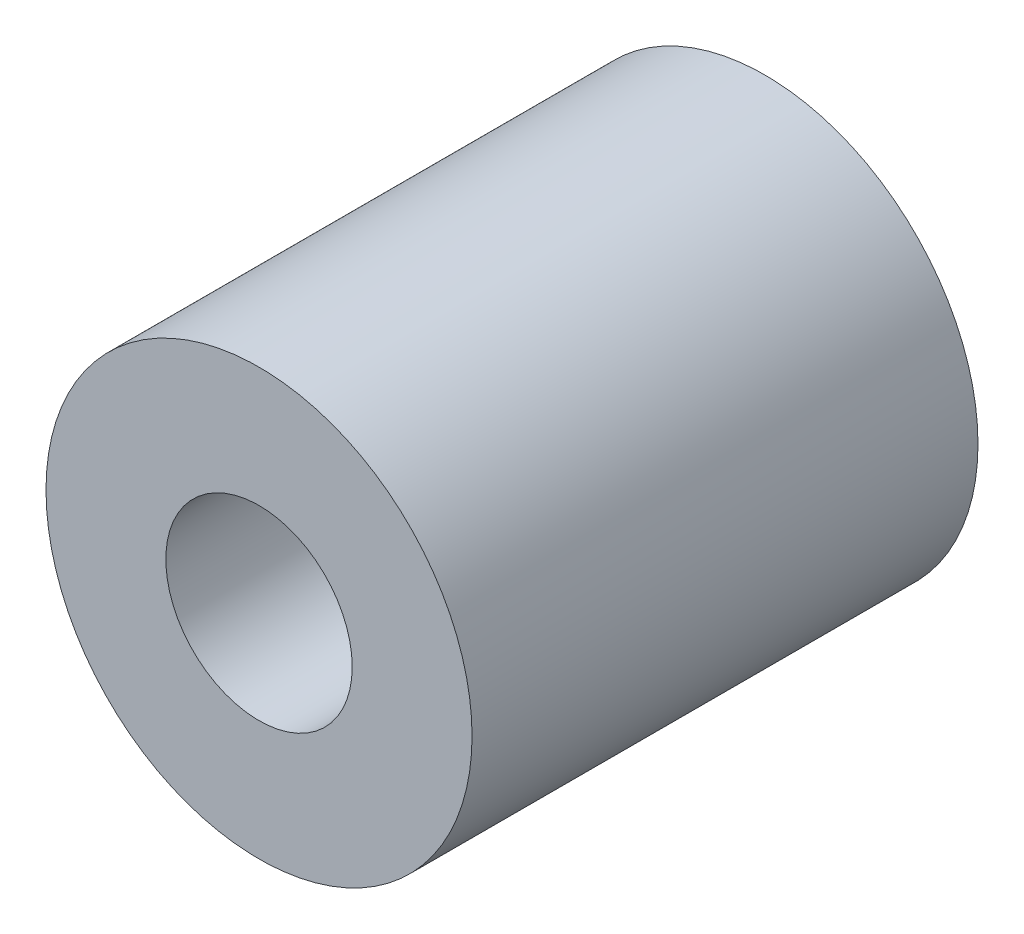
SolidWorks part; units mm, degrees
material "SS400B"
ref_plane "Front Plane" through (0, 0, 0) normal (0, 0, 1) x (1, 0, 0)
ref_plane "Top Plane" through (0, 0, 0) normal (0, 1, 0) x (1, 0, 0)
ref_plane "Right Plane" through (0, 0, 0) normal (1, 0, 0) x (0, 0, -1)
sketch "Sketch1" plane through (0, 0, 0) normal (0, 0, 1) x (1, 0, 0)
  circle A0 centre (0, 0) radius 16
  dimension "D1" = 32
extrude "Boss-Extrude1" add sketch "Sketch1" along normal blind 38
hole_wizard "M16 Tapped Hole1" positions "Sketch2" profile "Sketch3" tap size "M16" standard "GB" end condition through all
sketch "Sketch2" plane through (0, 0, 38) normal (0, 0, 1) x (1, 0, 0)
  point P0 (0, 0)
sketch "Sketch3" plane through (0, 0, 38) normal (1, 0, 0) x (0, -1, 0)
  line L0 (0, 0) -> (0, 38)
  line L1 (0, 38) -> (7, 38)
  line L2 (7, 38) -> (7, 0)
  line L5 (7, 0) -> (0, 0)
  line L11 (0, -6.35) -> (0, 107.95) construction
  dimension "通孔螺纹孔钻头直径" = 14
  dimension "通孔螺纹孔钻头深度" = 38
cosmetic thread "Hole Cosmetic Thread1" parameters "D2"=16
